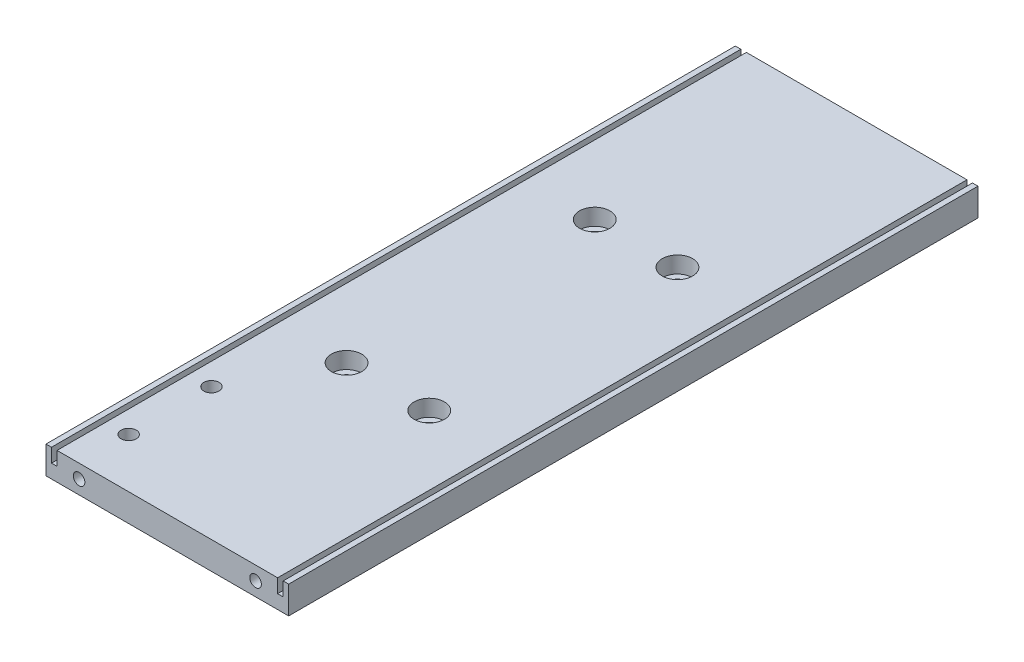
from build123d import *

# Parameters (mm, degrees)
SKETCH_1_W             = 88
SKETCH_1_H             = 10
EXTRUDE_1_DEPTH        = 250
SKETCH_2_W             = 2
SKETCH_2_H             = 5
CUT_EXTRUDE_1_DEPTH    = 254.891709199
HOLE_WIZARD_M5_1_D     = 4.2
HOLE_WIZARD_M5_1_DEPTH = 10
HOLE_WIZARD_M5_1_TIP   = 1.2618073
HOLE_WIZARD_M5_2_D     = 4.2
HOLE_WIZARD_M5_2_DEPTH = 10
HOLE_WIZARD_M5_2_TIP   = 1.2618073
SKETCH_7_R             = 3.25
CUT_EXTRUDE_2_DEPTH    = 255.039367028
SKETCH_8_R             = 5.5
CUT_EXTRUDE_3_DEPTH    = 6
SKETCH_9_R             = 2.75
CUT_EXTRUDE_4_DEPTH    = 255.039367028
SKETCH_10_R            = 4.5
CUT_EXTRUDE_5_DEPTH    = 5


with BuildPart() as part:
    # 草图1 → 凸台-拉伸1 (new body)
    with BuildSketch(Plane.XY):
        Rectangle(SKETCH_1_W, SKETCH_1_H)
    extrude(amount=EXTRUDE_1_DEPTH)

    # 草图2 → 切除-拉伸1 (cut, through all)
    with BuildSketch(Plane.XY.offset(250)):
        with Locations((-41, 2.5)):
            Rectangle(SKETCH_2_W, SKETCH_2_H)
        with Locations((41, 2.5)):
            Rectangle(SKETCH_2_W, SKETCH_2_H)
    extrude(amount=-CUT_EXTRUDE_1_DEPTH, mode=Mode.SUBTRACT)

    # M5 螺纹孔1
    with Locations(Plane(origin=(-32, 0, 250), x_dir=(1, 0, 0), z_dir=(0, 0, 1))):
        with Locations((0, 0), (64, 0)):
            Hole(HOLE_WIZARD_M5_1_D / 2, depth=HOLE_WIZARD_M5_1_DEPTH)
            with Locations((0, 0, -(HOLE_WIZARD_M5_1_DEPTH + HOLE_WIZARD_M5_1_TIP / 2))):  # 118° drill point
                Cone(0, HOLE_WIZARD_M5_1_D / 2, HOLE_WIZARD_M5_1_TIP, mode=Mode.SUBTRACT)

    # M5 螺纹孔2
    with Locations(Plane(origin=(32, 0, 0), x_dir=(-1, 0, 0), z_dir=(0, 0, -1))):
        with Locations((0, 0), (64, 0)):
            Hole(HOLE_WIZARD_M5_2_D / 2, depth=HOLE_WIZARD_M5_2_DEPTH)
            with Locations((0, 0, -(HOLE_WIZARD_M5_2_DEPTH + HOLE_WIZARD_M5_2_TIP / 2))):  # 118° drill point
                Cone(0, HOLE_WIZARD_M5_2_D / 2, HOLE_WIZARD_M5_2_TIP, mode=Mode.SUBTRACT)

    # 草图7 → 切除-拉伸2 (cut, through all)
    with BuildSketch(Plane(origin=(0, 5, 0), x_dir=(1, 0, 0), z_dir=(0, 1, 0))):
        with Locations(Location((-15, -80, 0), (0, 0, 270))):
            Circle(SKETCH_7_R)
        with Locations(Location((15, -80, 0), (0, 0, 270))):
            Circle(SKETCH_7_R)
        with Locations(Location((15, -170, 0), (0, 0, 90))):
            Circle(SKETCH_7_R)
        with Locations(Location((-15, -170, 0), (0, 0, 90))):
            Circle(SKETCH_7_R)
    extrude(amount=-CUT_EXTRUDE_2_DEPTH, mode=Mode.SUBTRACT)

    # 草图8 → 切除-拉伸3 (cut)
    with BuildSketch(Plane(origin=(0, 5, 0), x_dir=(1, 0, 0), z_dir=(0, 1, 0))):
        with Locations(Location((-15, -80, 0), (0, 0, 270))):
            Circle(SKETCH_8_R)
        with Locations(Location((15, -80, 0), (0, 0, 270))):
            Circle(SKETCH_8_R)
        with Locations(Location((-15, -170, 0), (0, 0, 270))):
            Circle(SKETCH_8_R)
        with Locations(Location((15, -170, 0), (0, 0, 270))):
            Circle(SKETCH_8_R)
    extrude(amount=-CUT_EXTRUDE_3_DEPTH, mode=Mode.SUBTRACT)

    # 草图9 → 切除-拉伸4 (cut, through all)
    with BuildSketch(Plane.XZ.offset(5)):
        with Locations(Location((-32, 232, 0), (0, 0, 270))):
            Circle(SKETCH_9_R)
        with Locations(Location((-32, 202, 0), (0, 0, 270))):
            Circle(SKETCH_9_R)
    extrude(amount=-CUT_EXTRUDE_4_DEPTH, mode=Mode.SUBTRACT)

    # 草图10 → 切除-拉伸5 (cut)
    with BuildSketch(Plane.XZ.offset(5)):
        with Locations(Location((-32, 232, 0), (0, 0, 270))):
            Circle(SKETCH_10_R)
        with Locations(Location((-32, 202, 0), (0, 0, 270))):
            Circle(SKETCH_10_R)
    extrude(amount=-CUT_EXTRUDE_5_DEPTH, mode=Mode.SUBTRACT)


solid = part.part
